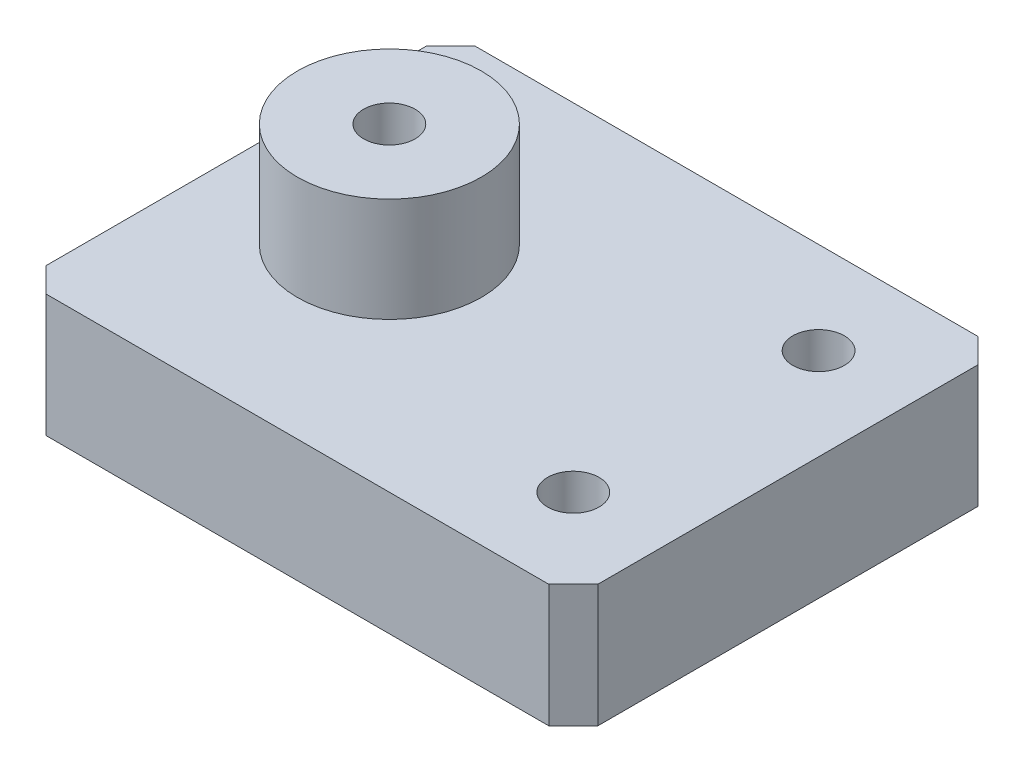
SolidWorks part; units mm, degrees
material "A6061"
ref_plane "前基準面" through (0, 0, 0) normal (0, 0, 1) x (1, 0, 0)
ref_plane "上基準面" through (0, 0, 0) normal (0, 1, 0) x (1, 0, 0)
ref_plane "右基準面" through (0, 0, 0) normal (1, 0, 0) x (0, 0, -1)
sketch "草图1" plane through (0, 0, 0) normal (0, 1, 0) x (1, 0, 0)
  line L1 (-22.5, -17.5) -> (22.5, -17.5)
  line L2 (-22.5, -17.5) -> (-22.5, 17.5)
  line L3 (-22.5, 17.5) -> (22.5, 17.5)
  line L4 (22.5, -17.5) -> (22.5, 17.5)
  line L5 (-22.5, -17.5) -> (22.5, 17.5) construction
  line L6 (-22.5, 17.5) -> (22.5, -17.5) construction
  point P0 (0, 0)
  dimension "D1" = 45
  dimension "D2" = 35
extrude "凸台-拉伸1" add sketch "草图1" along normal mid plane 10
sketch "草图2" plane through (0, 5, 0) normal (0, 1, 0) x (1, 0, 0)
  line L0 (-22.5, -17.5) -> (22.5, -17.5) construction
  line L1 (-22.5, -17.5) -> (7.5, -17.5)
  line L2 (-22.5, -17.5) -> (-22.5, 17.5)
  line L3 (-22.5, 17.5) -> (7.5, 17.5)
  line L4 (7.5, -17.5) -> (7.5, 17.5)
  line L5 (-22.5, 17.5) -> (-22.5, -17.5) construction
  line L6 (22.5, 17.5) -> (-22.5, 17.5) construction
  line L7 (22.5, -17.5) -> (22.5, 17.5) construction
  dimension "D1" = 15
extrude "切除-拉伸1" [suppressed] cut sketch "草图2" against normal blind 10
chamfer "倒角1" distance 2 angle 45 4 edges at (22.5, 0, 17.5) (22.5, 0, -17.5) (-22.5, 0, 17.5) (-22.5, 0, -17.5)
sketch "草图8" plane through (0, 5, 0) normal (0, 1, 0) x (1, 0, 0)
  line L0 (-22.5, 15.5) -> (-22.5, -15.5) construction
  circle A0 centre (-10, 0) radius 7.5
  dimension "D1" = 15
  dimension "D2" = 12.5
extrude "凸台-拉伸2" add sketch "草图8" along normal blind 8.5
hole_wizard "M5 螺纹孔1" positions "草图3" profile "草图5" tap size "M5" standard "GB" end condition through all
sketch "草图3" plane through (0, 5, 0) normal (0, 1, 0) x (1, 0, 0)
  line L0 (22.5, 0) -> (7.5, 0) construction
  line L1 (22.5, -15.5) -> (22.5, 15.5) construction
  line L4 (15, 0) -> (15, -5.7696) construction
  point P0 (15, -10)
  point P11 (15, 10)
  dimension "D1" = 20
  dimension "D2" = 7.5
sketch "草图5" plane through (15, 5, 10) normal (1, 0, 0) x (0, 0, 1)
  line L0 (0, 0) -> (0, 10)
  line L1 (0, 10) -> (2.1, 10)
  line L2 (2.1, 10) -> (2.1, 0)
  line L5 (2.1, 0) -> (0, 0)
  line L11 (0, -6.35) -> (0, 107.95) construction
  dimension "通孔螺纹孔钻头直径" = 4.2
  dimension "通孔螺纹孔钻头深度" = 10
cosmetic thread "孔螺蚊线1"
cosmetic thread "孔螺蚊线2"
hole_wizard "M5 螺纹孔2" positions "草图6" profile "草图7" tap size "M5" standard "GB" end condition through all
sketch "草图6" plane through (0, 13.5, 0) normal (0, 1, 0) x (1, 0, 0)
  line L1 (-22.5, 15.5) -> (-22.5, -15.5) construction
  point P0 (-10, 0)
  dimension "D1" = 12.5
cosmetic thread "孔螺蚊线4" parameters "D2"=5
sketch "草图7" plane through (-10, 13.5, 0) normal (1, 0, 0) x (0, 0, 1)
  line L0 (0, 0) -> (0, 18.5)
  line L1 (0, 18.5) -> (2.1, 18.5)
  line L2 (2.1, 18.5) -> (2.1, 0)
  line L5 (2.1, 0) -> (0, 0)
  line L11 (0, -6.35) -> (0, 107.95) construction
  dimension "通孔螺纹孔钻头直径" = 4.2
  dimension "通孔螺纹孔钻头深度" = 18.5
